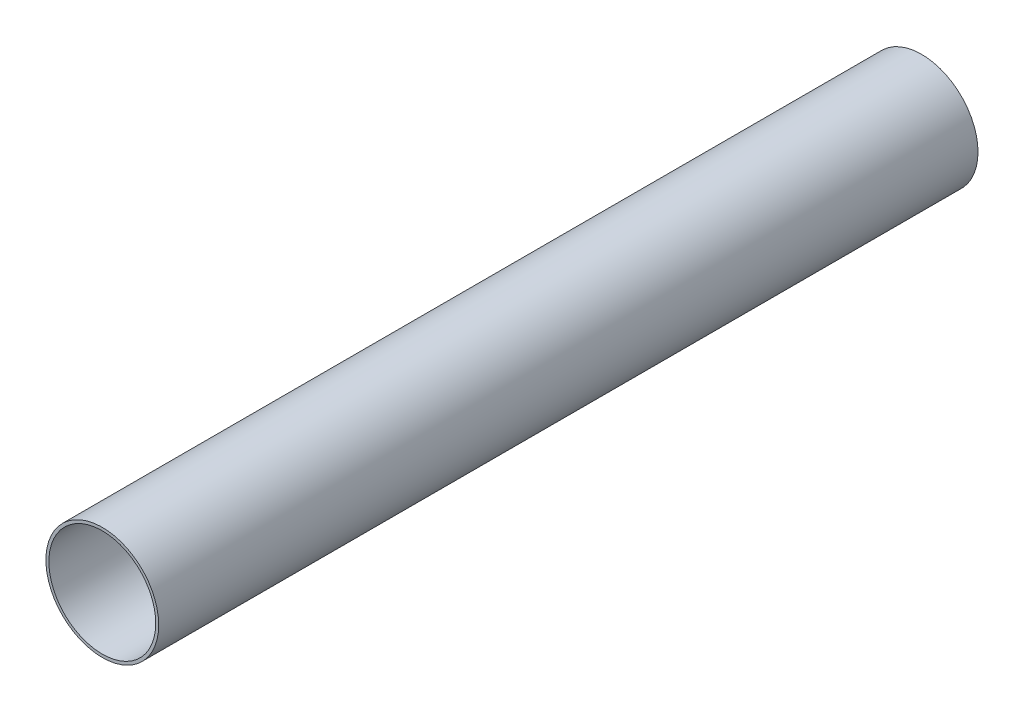
SolidWorks part; units mm, degrees
ref_plane "前视基准面" through (0, 0, 0) normal (0, 0, 1) x (1, 0, 0)
ref_plane "上视基准面" through (0, 0, 0) normal (0, 1, 0) x (1, 0, 0)
ref_plane "右视基准面" through (0, 0, 0) normal (1, 0, 0) x (0, 0, -1)
other "Configuration Table"
sketch "草图1" plane through (0, 0, 0) normal (0, 0, 1) x (1, 0, 0)
  circle A0 centre (0, 0) radius 45
  circle A1 centre (0, 0) radius 47.5
  dimension "D1" = 95
  dimension "D2" = 90
extrude "凸台-拉伸1" add sketch "草图1" along normal mid plane 690
